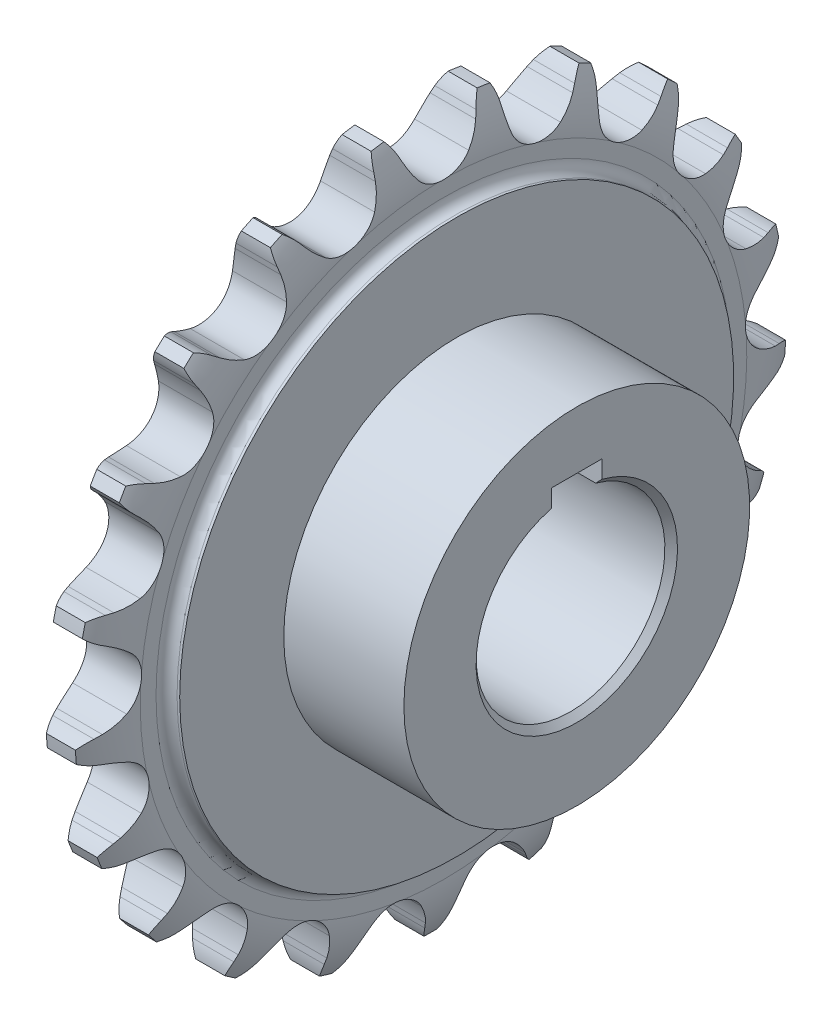
SolidWorks part; units mm, degrees
ref_plane "前视基准面" through (0, 0, 0) normal (0, 0, 1) x (1, 0, 0)
ref_plane "上视基准面" through (0, 0, 0) normal (0, 1, 0) x (1, 0, 0)
ref_plane "右视基准面" through (0, 0, 0) normal (1, 0, 0) x (0, 0, -1)
sketch "草图1" plane through (0, 0, 0) normal (0, 0, 1) x (1, 0, 0)
  line L0 (-7.9375, 0) -> (7.9375, 0) construction
  line L1 (-6.4594, 15) -> (-6.4594, 44)
  line L2 (-6.4594, 44) -> (-6.0417, 44)
  line L3 (-4.371, 45.6707) -> (-4.371, 48.1767)
  line L4 (-2.3072, 56.5) -> (2.3072, 56.5)
  line L5 (4.371, 48.1767) -> (4.371, 45.6707)
  line L6 (6.0417, 44) -> (6.4594, 44)
  line L7 (6.4594, 44) -> (6.4594, 15)
  line L8 (6.4594, 15) -> (-6.4594, 15)
  line L9 (0, 0) -> (0, 56.5) construction
  line L10 (-3.6982, 53.2567) -> (3.6982, 53.2567) construction
  line L11 (-3.6982, -53.2567) -> (3.6982, -53.2567) construction
  line L12 (7.9375, 0) -> (28.9375, 0) construction
  line L13 (-4.371, 48.1767) -> (3.7984, 48.1767) construction
  line L14 (-4.371, -48.1767) -> (3.7984, -48.1767) construction
  line L15 (28.9375, 0) -> (39.0975, 0) construction
  line L16 (39.0975, 0) -> (54.1875, 0) construction
  line L17 (54.1875, 0) -> (63.5875, 0) construction
  line L18 (63.5875, 0) -> (81.6975, 0) construction
  arc A0 (-2.3072, 56.5) -> (-4.371, 48.1767) centre (11.4966, 48.6598) ccw
  arc A1 (2.3072, 56.5) -> (4.371, 48.1767) centre (-11.4966, 48.6598) cw
  arc A2 (4.371, 45.6707) -> (6.0417, 44) centre (6.0417, 45.6707) ccw
  arc A3 (-6.0417, 44) -> (-4.371, 45.6707) centre (-6.0417, 45.6707) ccw
  point P30 (4.371, 44)
  point P33 (-4.371, 44)
  dimension "D1" = 4.1767
  dimension "rx" = 15.875
  dimension "D3" = 1.6707
  dimension "d" = 106.5134
  dimension "p" = 15.875
  dimension "z" = 21
  dimension "da" = 113
  dimension "df" = 96.3534
  dimension "dr" = 10.16
  dimension "dk" = 30
  dimension "dg" = 88
  dimension "h" = 15.09
  dimension "bf1" = 8.742
  dimension "b1" = 9.4
  dimension "ba" = 2.0638
  dimension "D2" = 2.0884
  dimension "pt" = 18.11
revolve "旋转1" add sketch "草图1" angle 360 about L0
sketch "草图2" plane through (0, 0, 0) normal (1, 0, 0) x (0, 0, -1)
  line L0 (0, 0) -> (0, 56.5) construction
  line L1 (0, 0) -> (-8.4209, 55.8689) construction
  line L2 (0, 0) -> (-16.6537, 53.9899) construction
  line L3 (4.0704, 50.0929) -> (10.2701, 45.274) construction
  line L4 (5.8527, 53.1564) -> (-6.4174, 58.2448) construction
  line L5 (0, 0) -> (8.4209, 55.8689) construction
  line L6 (5.8527, 53.1564) -> (6.2493, 54.1127)
  line L7 (-5.8527, 53.1564) -> (-6.2493, 54.1127)
  circle A0 centre (0, 0) radius 56.5 construction
  arc A1 (4.0704, 50.0929) -> (-4.0704, 50.0929) centre (0, 53.2567) cw
  arc A2 (4.0704, 50.0929) -> (5.8527, 53.1564) centre (-6.4174, 58.2448) ccw
  arc A3 (7.3999, 56.0133) -> (6.2493, 54.1127) centre (13.0605, 51.2882) ccw
  arc A4 (-4.0704, 50.0929) -> (-5.8527, 53.1564) centre (6.4174, 58.2448) cw
  arc A5 (-7.3999, 56.0133) -> (-6.2493, 54.1127) centre (-13.0605, 51.2882) cw
  arc A7 (7.3999, 56.0133) -> (-7.3999, 56.0133) centre (0, 0) ccw
  dimension "r1" = 5.1554
  dimension "r3" = 7.3736
  dimension "D1" = 17.143
  dimension "D2" = 8.571
  dimension "α/2" = 52.143
  dimension "M" = 6.4174
  dimension "T" = 4.9881
  dimension "β" = 15.333
  dimension "γ/2" = 13.952
  dimension "bc" = 1.0353
extrude "切除-拉伸1" cut sketch "草图2" against normal mid plane 12.9187
pattern_circular "阵列(圆周)1" count 21 over 360 about axis through (0, 0, 0) along (1, 0, 0) of "切除-拉伸1"
sketch "草图3" plane through (0, 0, 0) normal (0, 0, 1) x (1, 0, 0)
  line L0 (6.4594, 15) -> (25.5406, 15)
  line L3 (25.5406, 15) -> (25.5406, 27.4651)
  line L4 (25.5406, 27.4651) -> (6.4594, 27.4651)
  line L5 (6.4594, 27.4651) -> (6.4594, 15)
  line L6 (0, 0) -> (6.4, 0) construction
  line L8 (-6.4594, 44) -> (-6.4594, -44) construction
  dimension "h" = 12.4651
  dimension "K" = 6.4
  dimension "L" = 32
revolve "旋转2" add sketch "草图3" angle 360 about L6
sketch "草图4" plane through (-6.4594, 0, 0) normal (-1, 0, 0) x (0, 0, 1)
  line L1 (-4, 14.4568) -> (4, 14.4568)
  line L2 (-4, 14.4568) -> (-4, 18.3)
  line L3 (-4, 18.3) -> (4, 18.3)
  line L4 (4, 14.4568) -> (4, 18.3)
  circle A0 centre (0, 0) radius 15 construction
  point P6 (0.7, 18.3)
  dimension "D1" = 18.3
  dimension "键槽宽度" = 8
  dimension "t1" = 3.3
extrude "切除-拉伸2" cut sketch "草图4" against normal through all
chamfer "倒角1" distance 1 angle 45 1 edges at (-6.4594, -15, 0)
chamfer "倒角3" distance 1 angle 45 1 edges at (25.5406, -15, 0)
